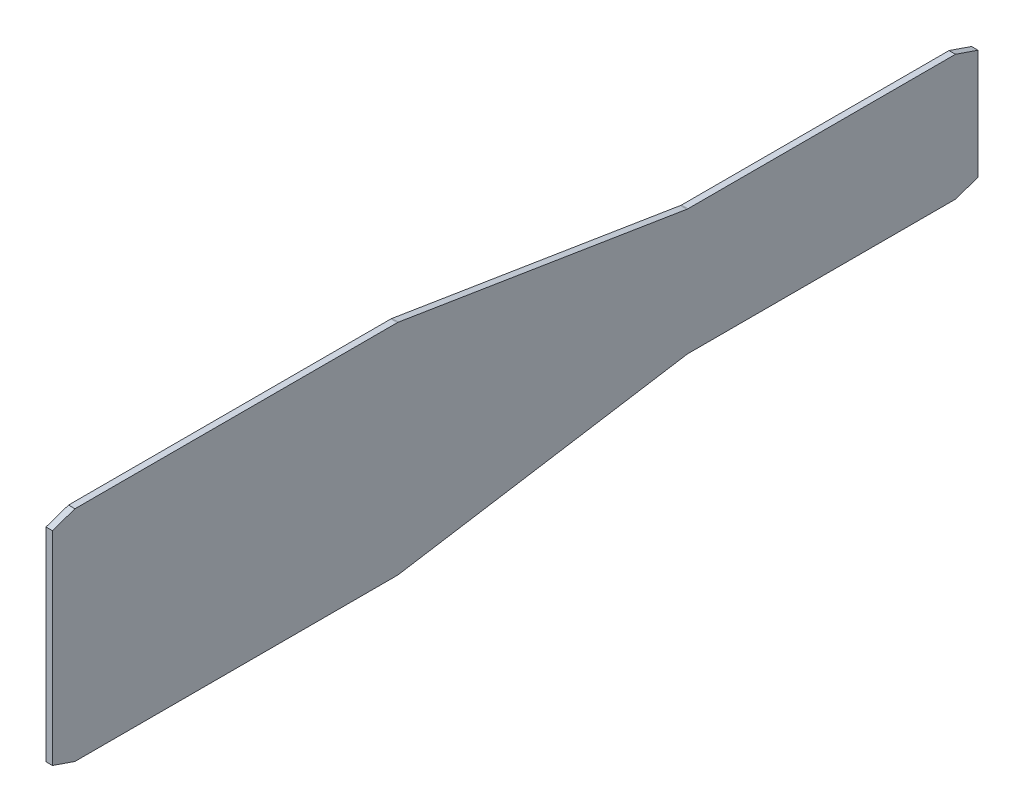
SolidWorks part; units mm, degrees
ref_plane "Front Plane" through (0, 0, 0) normal (0, 0, 1) x (1, 0, 0)
ref_plane "Top Plane" through (0, 0, 0) normal (0, 1, 0) x (1, 0, 0)
ref_plane "Right Plane" through (0, 0, 0) normal (1, 0, 0) x (0, 0, -1)
sketch "Sketch1" plane through (0, 0, 0) normal (1, 0, 0) x (0, 0, -1)
  line L0 (0, -158) -> (0, 158)
  line L1 (35, 170) -> (535.7996, 170)
  line L2 (537.3902, 169.8727) -> (985.8098, 97.6273)
  line L3 (987.4004, 97.5) -> (1403, 97.5)
  line L4 (1438, 85.5) -> (1438, -85.5)
  line L5 (0, 0) -> (1056.3772, 0) construction
  line L6 (0, 158) -> (35, 170)
  line L7 (1438, 85.5) -> (1403, 97.5)
  line L8 (1438, -85.5) -> (1403, -97.5)
  line L9 (987.4004, -97.5) -> (1403, -97.5)
  line L10 (537.3902, -169.8727) -> (985.8098, -97.6273)
  line L11 (0, -158) -> (35, -170)
  line L12 (35, -170) -> (535.7996, -170)
  arc A0 (987.4004, 97.5) -> (985.8098, 97.6273) centre (987.4004, 107.5) cw
  arc A1 (537.3902, 169.8727) -> (535.7996, 170) centre (535.7996, 160) ccw
  arc A2 (987.4004, -97.5) -> (985.8098, -97.6273) centre (987.4004, -107.5) ccw
  arc A3 (537.3902, -169.8727) -> (535.7996, -170) centre (535.7996, -160) cw
  point P12 (986.6, 97.5)
  point P15 (536.6, 170)
  point P17 (1438, 0)
  point P21 (986.6, -97.5)
  point P27 (536.6, -170)
  dimension "D10" = 10
  dimension "D1" = 1438
  dimension "D2" = 340
  dimension "D3" = 536.6
  dimension "D4" = 451.4
  dimension "D5" = 195
  dimension "D6" = 35
  dimension "D7" = 12
  dimension "D8" = 35
  dimension "D9" = 12
extrude "Boss-Extrude1" add sketch "Sketch1" along normal blind 10
